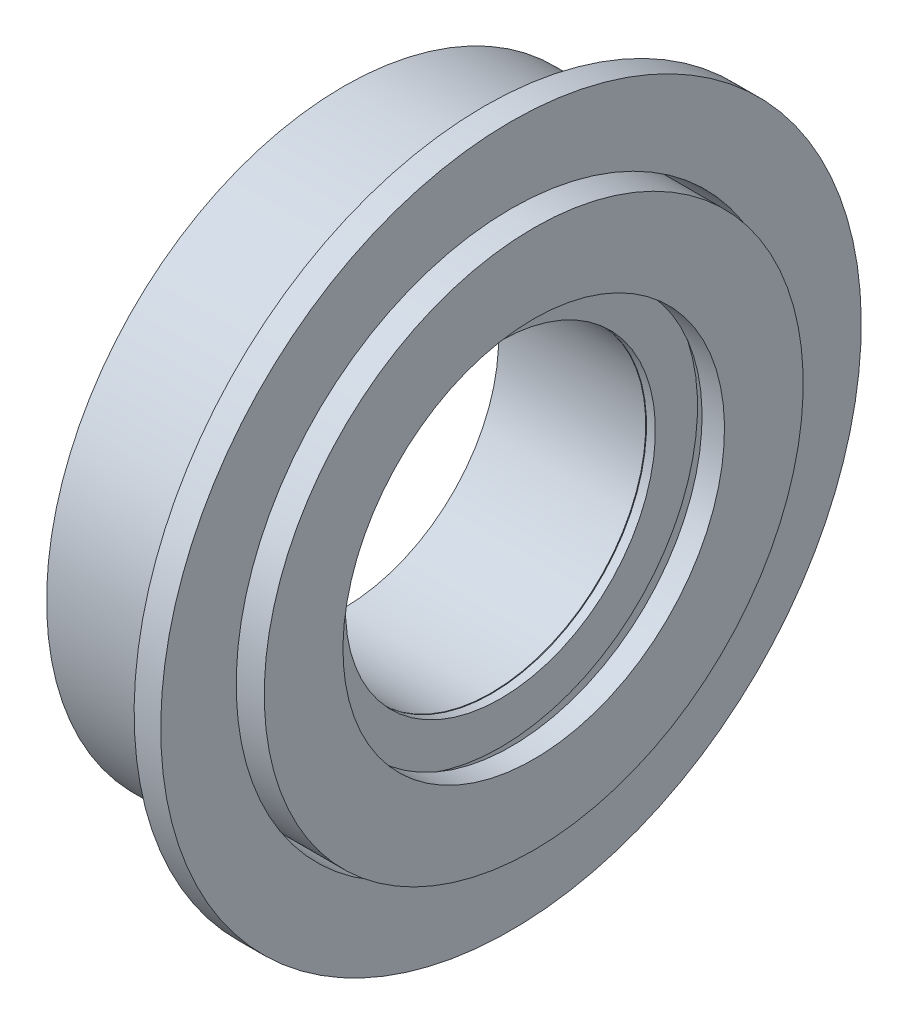
SolidWorks part; units mm, degrees
ref_plane "Front Plane" through (0, 0, 0) normal (0, 0, 1) x (1, 0, 0)
ref_plane "Top Plane" through (0, 0, 0) normal (0, 1, 0) x (1, 0, 0)
ref_plane "Right Plane" through (0, 0, 0) normal (1, 0, 0) x (0, 0, -1)
sketch "Sketch1" plane through (0, 0, 0) normal (0, 0, 1) x (1, 0, 0)
  line L0 (0, 0) -> (-16.6488, 0) construction
  line L1 (93, 39.4546) -> (93, 33.4546)
  line L2 (93, -56.011) -> (93, 56.011) construction
  line L3 (93, 39.4546) -> (93, -39.4546) construction
  line L4 (90, 33.4546) -> (74.1426, 33.4546)
  line L5 (74.1426, 33.4546) -> (74.1426, 17.4546)
  line L6 (74.1426, 17.4546) -> (90.7243, 17.4546)
  line L7 (90.7243, 17.4546) -> (90.7243, 20.4546)
  line L8 (90.7243, 20.4546) -> (77, 20.4546)
  line L9 (90, 33.4546) -> (90, 39.4546)
  line L10 (90, 39.4546) -> (93, 39.4546)
  line L11 (77, 20.4546) -> (77, 30.9546)
  line L12 (77, 30.9546) -> (93, 30.9546)
  line L13 (93, 30.9546) -> (93, 33.4546)
  line L14 (93, 33.4546) -> (92.9732, 33.4642)
  line L15 (77.8482, 30.3555) -> (92, 30.3555)
  line L16 (92, 55.3734) -> (92, -55.3734) construction
  line L18 (90.7243, 26.5741) -> (77.8482, 26.5741)
  line L19 (77.8482, 26.5741) -> (77.8482, 30.3555)
  line L20 (90.7217, 26.5719) -> (78.0969, 26.5719)
  line L21 (93.0345, 25.0021) -> (90.7243, 25.0021)
  line L22 (90.7243, 25.0021) -> (90.7243, 26.5741)
  line L23 (92, 30.3555) -> (95.561, 30.3555)
  line L24 (95.561, 30.3555) -> (95.561, 21.4896)
  line L25 (95.561, 21.4896) -> (93.0345, 21.4896)
  line L26 (93.0345, 21.4896) -> (93.0345, 25.0021)
  line L27 (90.7217, 26.5719) -> (90.7217, 20.4919)
  line L28 (90.7217, 20.4919) -> (78.0969, 20.4919)
  line L29 (78.0969, 26.5719) -> (78.0969, 20.4919)
  line L30 (90.8113, 22.1991) -> (91.8113, 22.1991)
  line L31 (90.8113, 22.1991) -> (90.8113, 17.4546)
  line L32 (90.8113, 17.4546) -> (91.8113, 17.4546)
  line L33 (91.8113, 22.1991) -> (91.8113, 17.4546)
revolve "Revolve1" add sketch "Sketch1" angle 360 about L0
